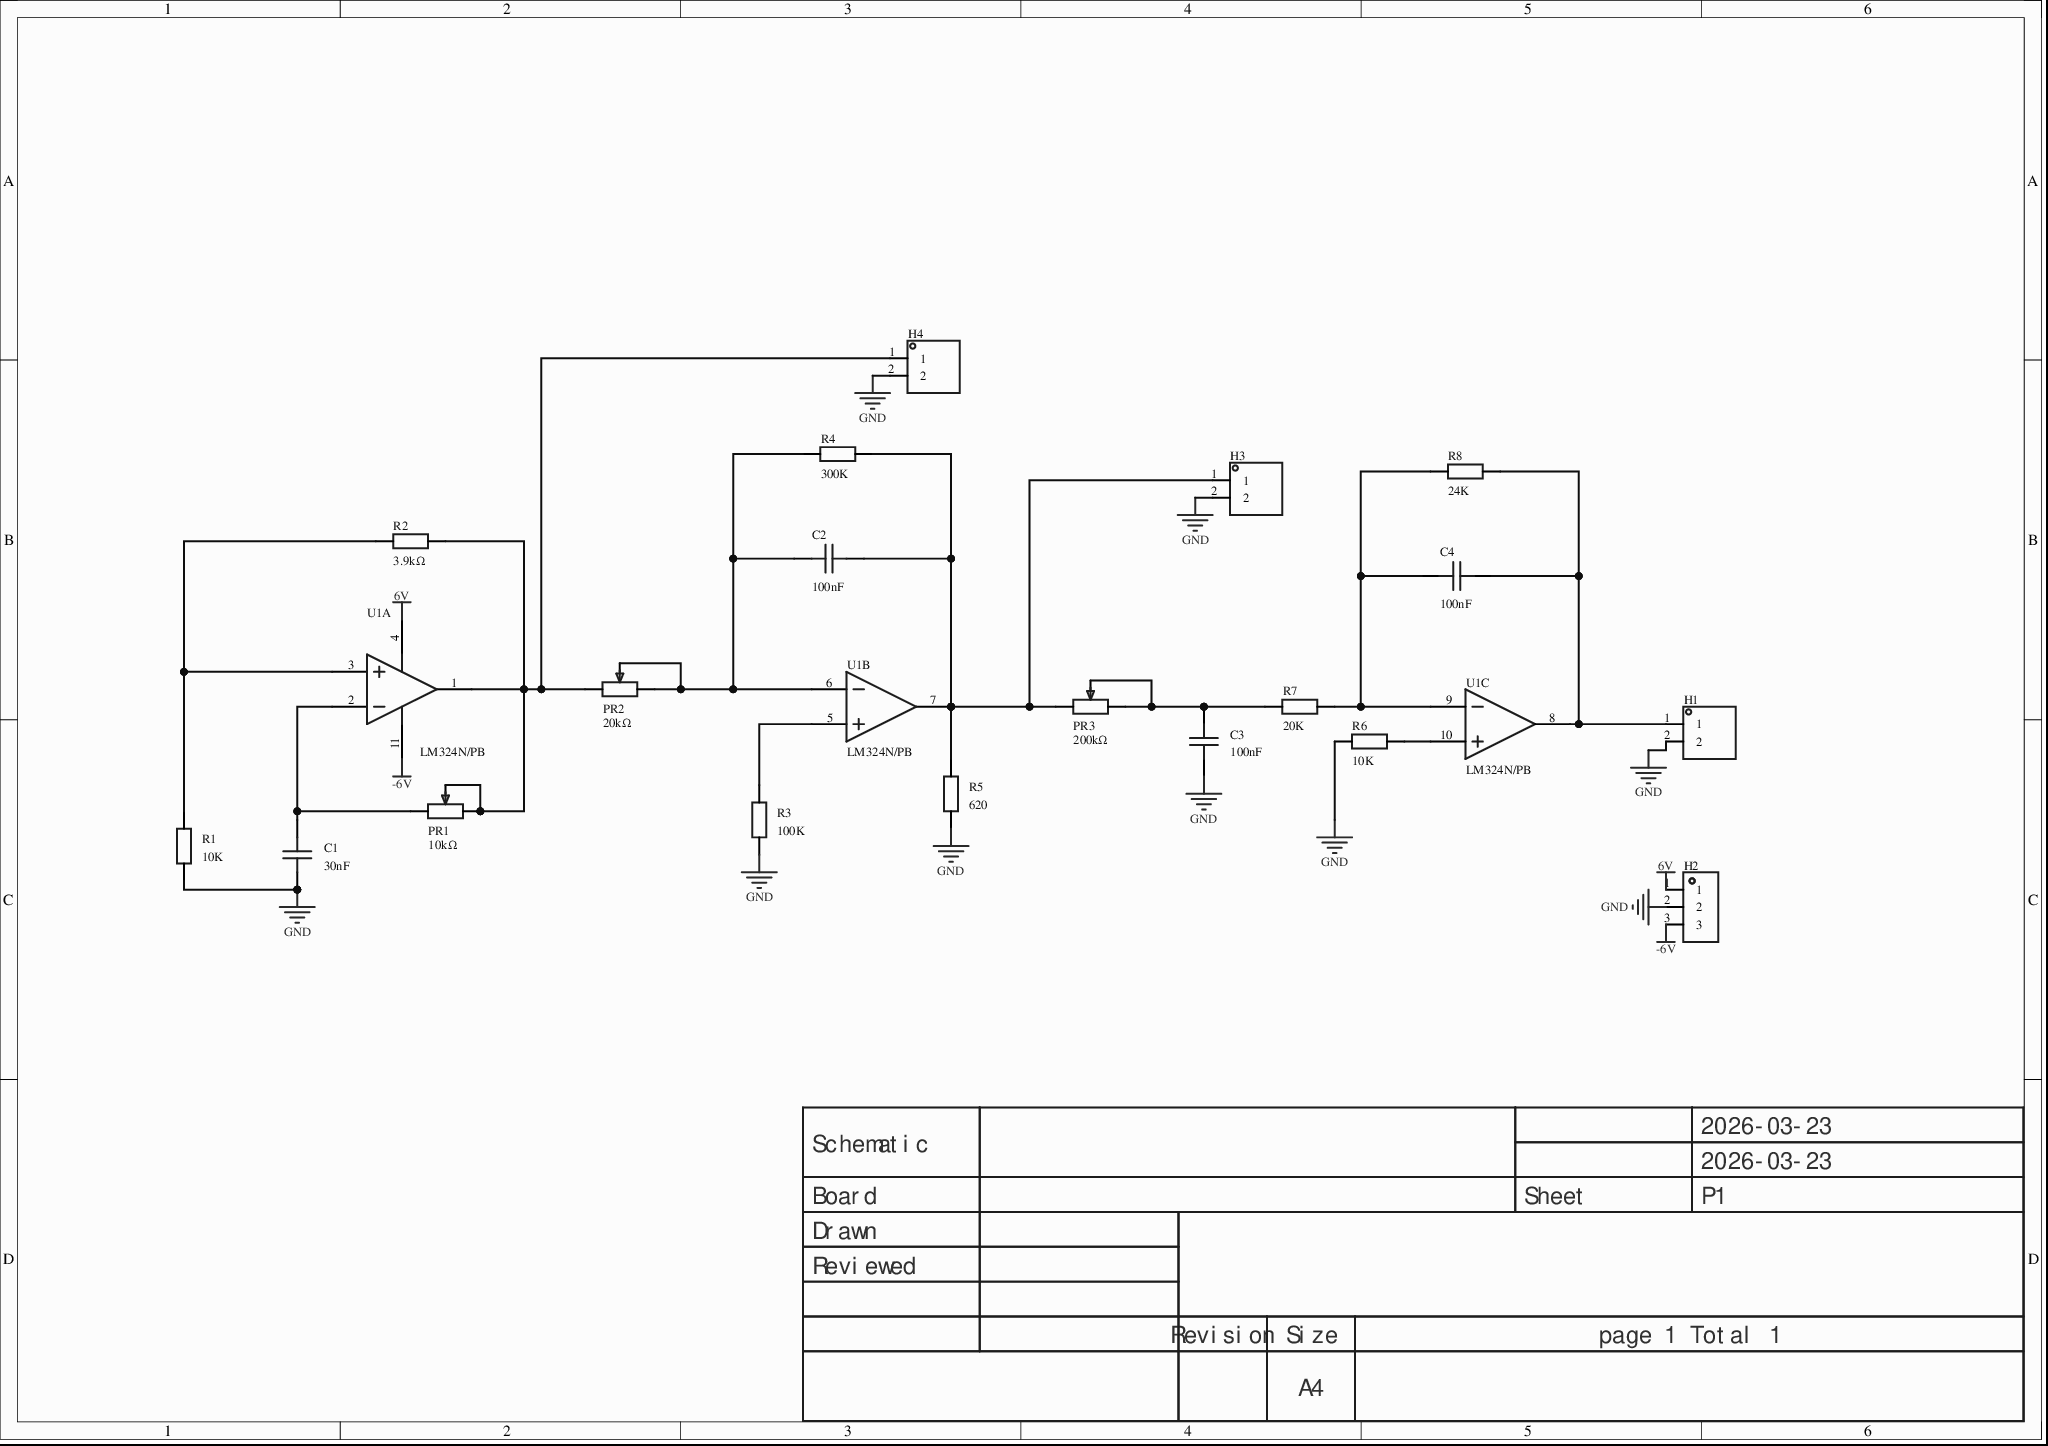
[diagram p0: MISC51897-3.schdoc]
# Altium project MISC51897-2.PrjPcb
1 sheet, 20 parts. Net scope: global (net labels, ports and power ports of the same name join across sheets).
Board file: MISC51897.pcbdoc

## Sheet MISC51897-3.schdoc
size 297 x 209 mm; Version: V1.0; @Project Name: MISC51897; @Update Date: 2026-03-23; @Create Date: 2026-03-23; @Board Name: MISC51897; @Create Time: 13:45:22; @Page Count: 1; @Page No: 1; @Schematic Name: MISC51897; @Update Time: 13:45:22; Size: A4

### Parts
C1  30nF  [C0603]
C2  100nF  [C0603]
C3  100nF  [C0603]
C4  100nF  [C0603]
H1  (no value)  [HDR-TH_2P-P2.54-V-M-1]
H2  (no value)  [HDR-TH_3P-P2.54-V-M]
H3  (no value)  [HDR-TH_2P-P2.54-V-M-1]
H4  (no value)  [HDR-TH_2P-P2.54-V-M-1]
PR1  10kΩ  [R_3296]
PR2  20kΩ  [R_3296]
PR3  200kΩ  [R_3296]
R1  10K  [R0603]
R2  3.9kΩ  [R0603]
R3  100K  [R0603]
R4  300K  [R0603]
R5  620  [R0603]
R6  10K  [R0603]
R7  20K  [R0603]
R8  24K  [R0603]
U1  LM324N/PB  [PDIP-14_L19.2-W6.6-P2.54-LS7.6-BL]  (parts A,B,C of 4)

### Nets
6V: H2.1 U1.4(V+)
-6V: H2.3 U1.11(GND)
GND: C1.1 C3.1 H1.2 H2.2 H3.2 H4.2 R1.1 R3.1 R5.1 R6.1
NetC1_2: C1.2 PR1.3 U1.2(INA+)
NetC2_1: C2.1 PR2.1 PR2.2 R4.1 U1.6(INB-)
NetC2_2: C2.2 H3.1 PR3.3 R4.2 R5.2 U1.7(OUTB)
NetC3_2: C3.2 PR3.1 PR3.2 R7.1
NetC4_1: C4.1 R7.2 R8.1 U1.9(INC-)
NetC4_2: C4.2 H1.1 R8.2 U1.8(OUTC)
NetH4_1: H4.1 PR1.1 PR1.2 PR2.3 R2.1 U1.1(OUTA)
NetR1_2: R1.2 R2.2 U1.3(INA-)
NetR3_2: R3.2 U1.5(INB+)
NetR6_2: R6.2 U1.10(INC+)

### Notes on the sheet
- 2026-03-23
- Schematic
- Board
- Sheet
- P1
- Drawn
- Reviewed
- Revision
- Size
- A4
- page 1 Total 1

### Library data of the parts
C1-C4 = CAP_0603: Symbol: Capacitance; ConvertToPcb: yes; ModelId: ac125912035d415993ca9572d50418b10819f05c4eef4c71ace90d822a990e87; ModelName: C0603_L1.6-W0.8-H0.8; ModelTransform: 62.992,31.496,0,0,0,0,0,0,0; Device: CAP_0603; AddInBom: yes; Supplier Footprint: 0603; FootprintName: C0603
  C1: Value: 30nF
  C2-C4: Value: 100nF
H1 H3 H4 = HDR-M_2.54_1x2P: Symbol: 210S-1*2P L=11.6MMGold-plated black; ConvertToPcb: yes; ModelId: 79b2e9f2d70a4d68a1b7098f27c6d4c50819f05c4eef4c71ace90d822a990e87; ModelName: HDR-M-2.54_1x2; ModelTransform: 200,100,0,0,0,0,0,0,-118.11; Device: HDR-M_2.54_1x2P; AddInBom: yes; SupplierPart: C124375; Supplier Footprint: 插件; FootprintName: HDR-TH_2P-P2.54-V-M-1
H2 = HDR-M_2.54_1x3P: AddInBom: yes; ModelId: bb473b6d38ff42a99216a4fcdbdcc4cb0819f05c4eef4c71ace90d822a990e87; ModelName: HDR-TH_3P-P2.54-M-LI-1X3P; ModelTransform: 300.03877,100,0,0,0,0,0,0,-118.11; Symbol: HDR-M_2.54_1x3P; Device: HDR-M_2.54_1x3P; ConvertToPcb: yes; FootprintName: HDR-TH_3P-P2.54-V-M; SupplierPart: C2937625; Supplier Footprint: 插件
PR1-PR3 = R_3296: ConvertToPcb: yes; ModelId: b182808559bb43bda9e7de64b64134cb0819f05c4eef4c71ace90d822a990e87; ModelName: 3296W; ModelTransform: 373.98,188.96,590.49,180,0,0,0,0,-140; Symbol: R_3296; Device: R_3296; AddInBom: yes; Supplier Footprint: 直插; FootprintName: R_3296
  PR1: Value: 10kΩ
  PR2: Value: 20kΩ
  PR3: Value: 200kΩ
R1-R8 = Res_0603: Symbol: Resistor; ConvertToPcb: yes; ModelId: fc143cca1e79419f9cd78b61e9279f080819f05c4eef4c71ace90d822a990e87; ModelTransform: 31.8897,63.7794,0,90,0,0,0,0,0; Device: Res_0603; AddInBom: yes; Supplier Footprint: 0603; FootprintName: R0603; ModelName: R0603
  R1 R6: Value: 10K
  R2: Value: 3.9kΩ
  R3: Value: 100K
  R4: Value: 300K
  R5: Value: 620
  R7: Value: 20K
  R8: Value: 24K
U1 = LM324N/PB: Amplifiers: quad; gain-bandwidth product (GBP): 1MHz; input bias current (Ib): 45nA;; Manufacturer: TI(德州仪器); Relevance: []; AddInBom: yes; ModelId: 08aeb3774ab0450ba412f07c9830bd710819f05c4eef4c71ace90d822a990e87; ModelTransform: 755.904,309.842,0,0,0,0,0,0,-129.921; Output Current: 40mA; Symbol: LM324N/PB; Device: LM324N/PB; LCSC Part Name: LM324N/PB; SupplierPart: C4366406; ManufacturerPart: LM324N/PB; Supplier Footprint: PDIP-14; JLCPCB Part Class: Extended Part; Datasheet: https://atta.szlcsc.com/upload/public/pdf/source/20230921/264342EF71D0FEA3F079F4D0F511985F.pdf; Supplier: LCSC; ConvertToPcb: yes; FootprintName: PDIP-14_L19.2-W6.6-P2.54-LS7.6-BL; ModelName: PDIP-14_L19.2-W6.6-P2.54-LS7.6-BL; Number of Circuits: Quad; Gain Bandwidth Product(GBP): 1MHz; Current - Input Bias(Ib): 45nA; Operating Temperature: 0℃~+70℃